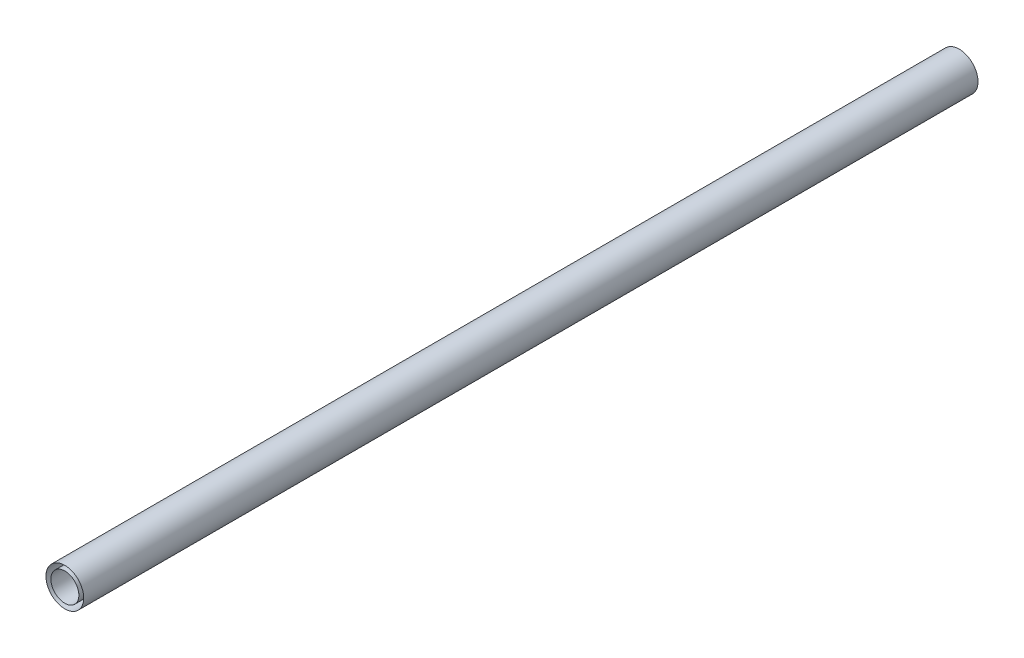
SolidWorks part; units mm, degrees
ref_plane "Front Plane" through (0, 0, 0) normal (0, 0, 1) x (1, 0, 0)
ref_plane "Top Plane" through (0, 0, 0) normal (0, 1, 0) x (1, 0, 0)
ref_plane "Right Plane" through (0, 0, 0) normal (1, 0, 0) x (0, 0, -1)
sketch "Sketch1" plane through (0, 0, 0) normal (0, 0, 1) x (1, 0, 0)
  circle A0 centre (0, 0) radius 95
  circle A1 centre (0, 0) radius 94.975
  dimension "D1" = 190
  dimension "D2" = 189.95
extrude "Boss-Extrude1" add sketch "Sketch1" along normal blind 4500
sketch "Sketch2" plane through (0, 0, 0) normal (0, 0, 1) x (1, 0, 0)
  circle A0 centre (0, 0) radius 70.5
  circle A1 centre (0, 0) radius 70.475
  dimension "D1" = 141
  dimension "D2" = 140.95
extrude "Boss-Extrude2" add sketch "Sketch2" along normal blind 4500 separate body
